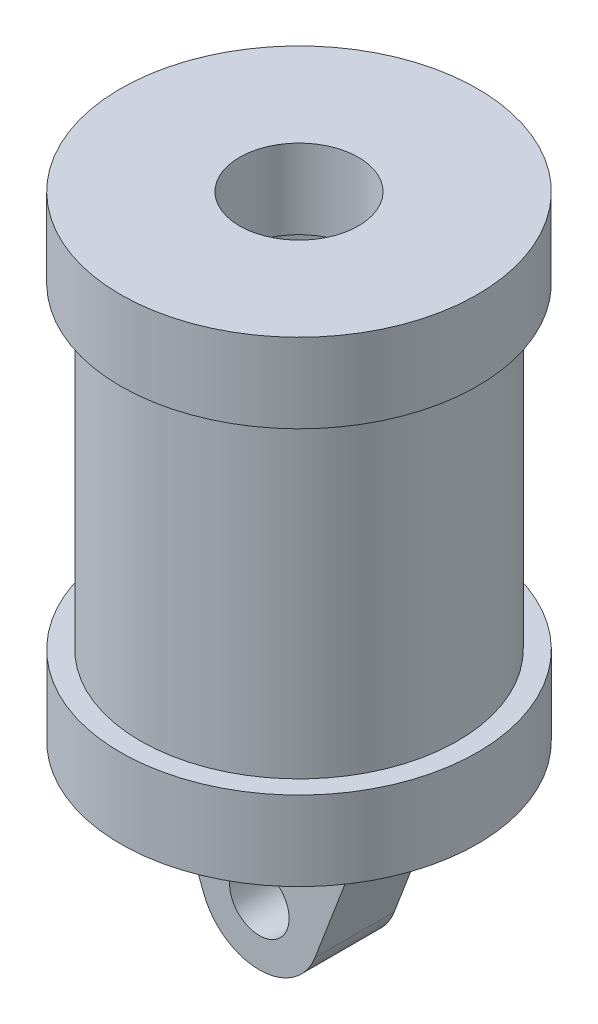
SolidWorks part; units mm, degrees
material "铸造碳钢"
ref_plane "前视基准面" through (0, 0, 0) normal (0, 0, 1) x (1, 0, 0)
ref_plane "上视基准面" through (0, 0, 0) normal (0, 1, 0) x (1, 0, 0)
ref_plane "右视基准面" through (0, 0, 0) normal (1, 0, 0) x (0, 0, -1)
sketch "草图1" plane through (0, 0, 0) normal (0, 1, 0) x (1, 0, 0)
  circle A0 centre (0, 0) radius 40
  dimension "D1" = 80
extrude "凸台-拉伸1" add sketch "草图1" along normal blind 80
sketch "草图2" plane through (0, 0, 0) normal (0, -1, 0) x (1, 0, 0)
  circle A2 centre (0, 0) radius 45
  dimension "D1" = 90
extrude "凸台-拉伸2" add sketch "草图2" along normal blind 20
sketch "草图3" plane through (0, 80, 0) normal (0, 1, 0) x (1, 0, 0)
  circle A0 centre (0, 0) radius 45
  dimension "D1" = 90
extrude "凸台-拉伸3" add sketch "草图3" along normal blind 20
sketch "草图4" plane through (0, 100, 0) normal (0, 1, 0) x (1, 0, 0)
  circle A0 centre (0, 0) radius 30
  dimension "D1" = 60
extrude "切除-拉伸2" cut sketch "草图4" against normal blind 80 from offset 20 offset against normal yes
sketch "草图5" plane through (0, 100, 0) normal (0, 1, 0) x (1, 0, 0)
  circle A0 centre (0, 0) radius 15
  dimension "D1" = 30
extrude "切除-拉伸3" cut sketch "草图5" against normal blind 40
sketch "草图6" plane through (0, 0, 0) normal (0, 0, 1) x (1, 0, 0)
  line L0 (-14.0147, -55.3468) -> (-27.5, -20)
  line L1 (-45, -20) -> (45, -20) construction
  line L2 (14.0147, -55.3468) -> (27.5, -20)
  line L3 (0, -72.1825) -> (0, 72.1825) construction
  line L4 (-27.5, -20) -> (27.5, -20)
  circle A0 centre (0, -50) radius 7.5
  arc A1 (-14.0147, -55.3468) -> (14.0147, -55.3468) centre (0, -50) ccw
  point P13 (0, 0)
  dimension "D2" = 15
  dimension "D3" = 30
  dimension "D1" = 30
  dimension "D4" = 55
extrude "凸台-拉伸4" add sketch "草图6" along normal mid plane 20
fillet "圆角1" radius 2 4 edges at (0, -20, -10) (27.5, -20, 0) (-27.5, -20, 0) (0, -20, 10)
